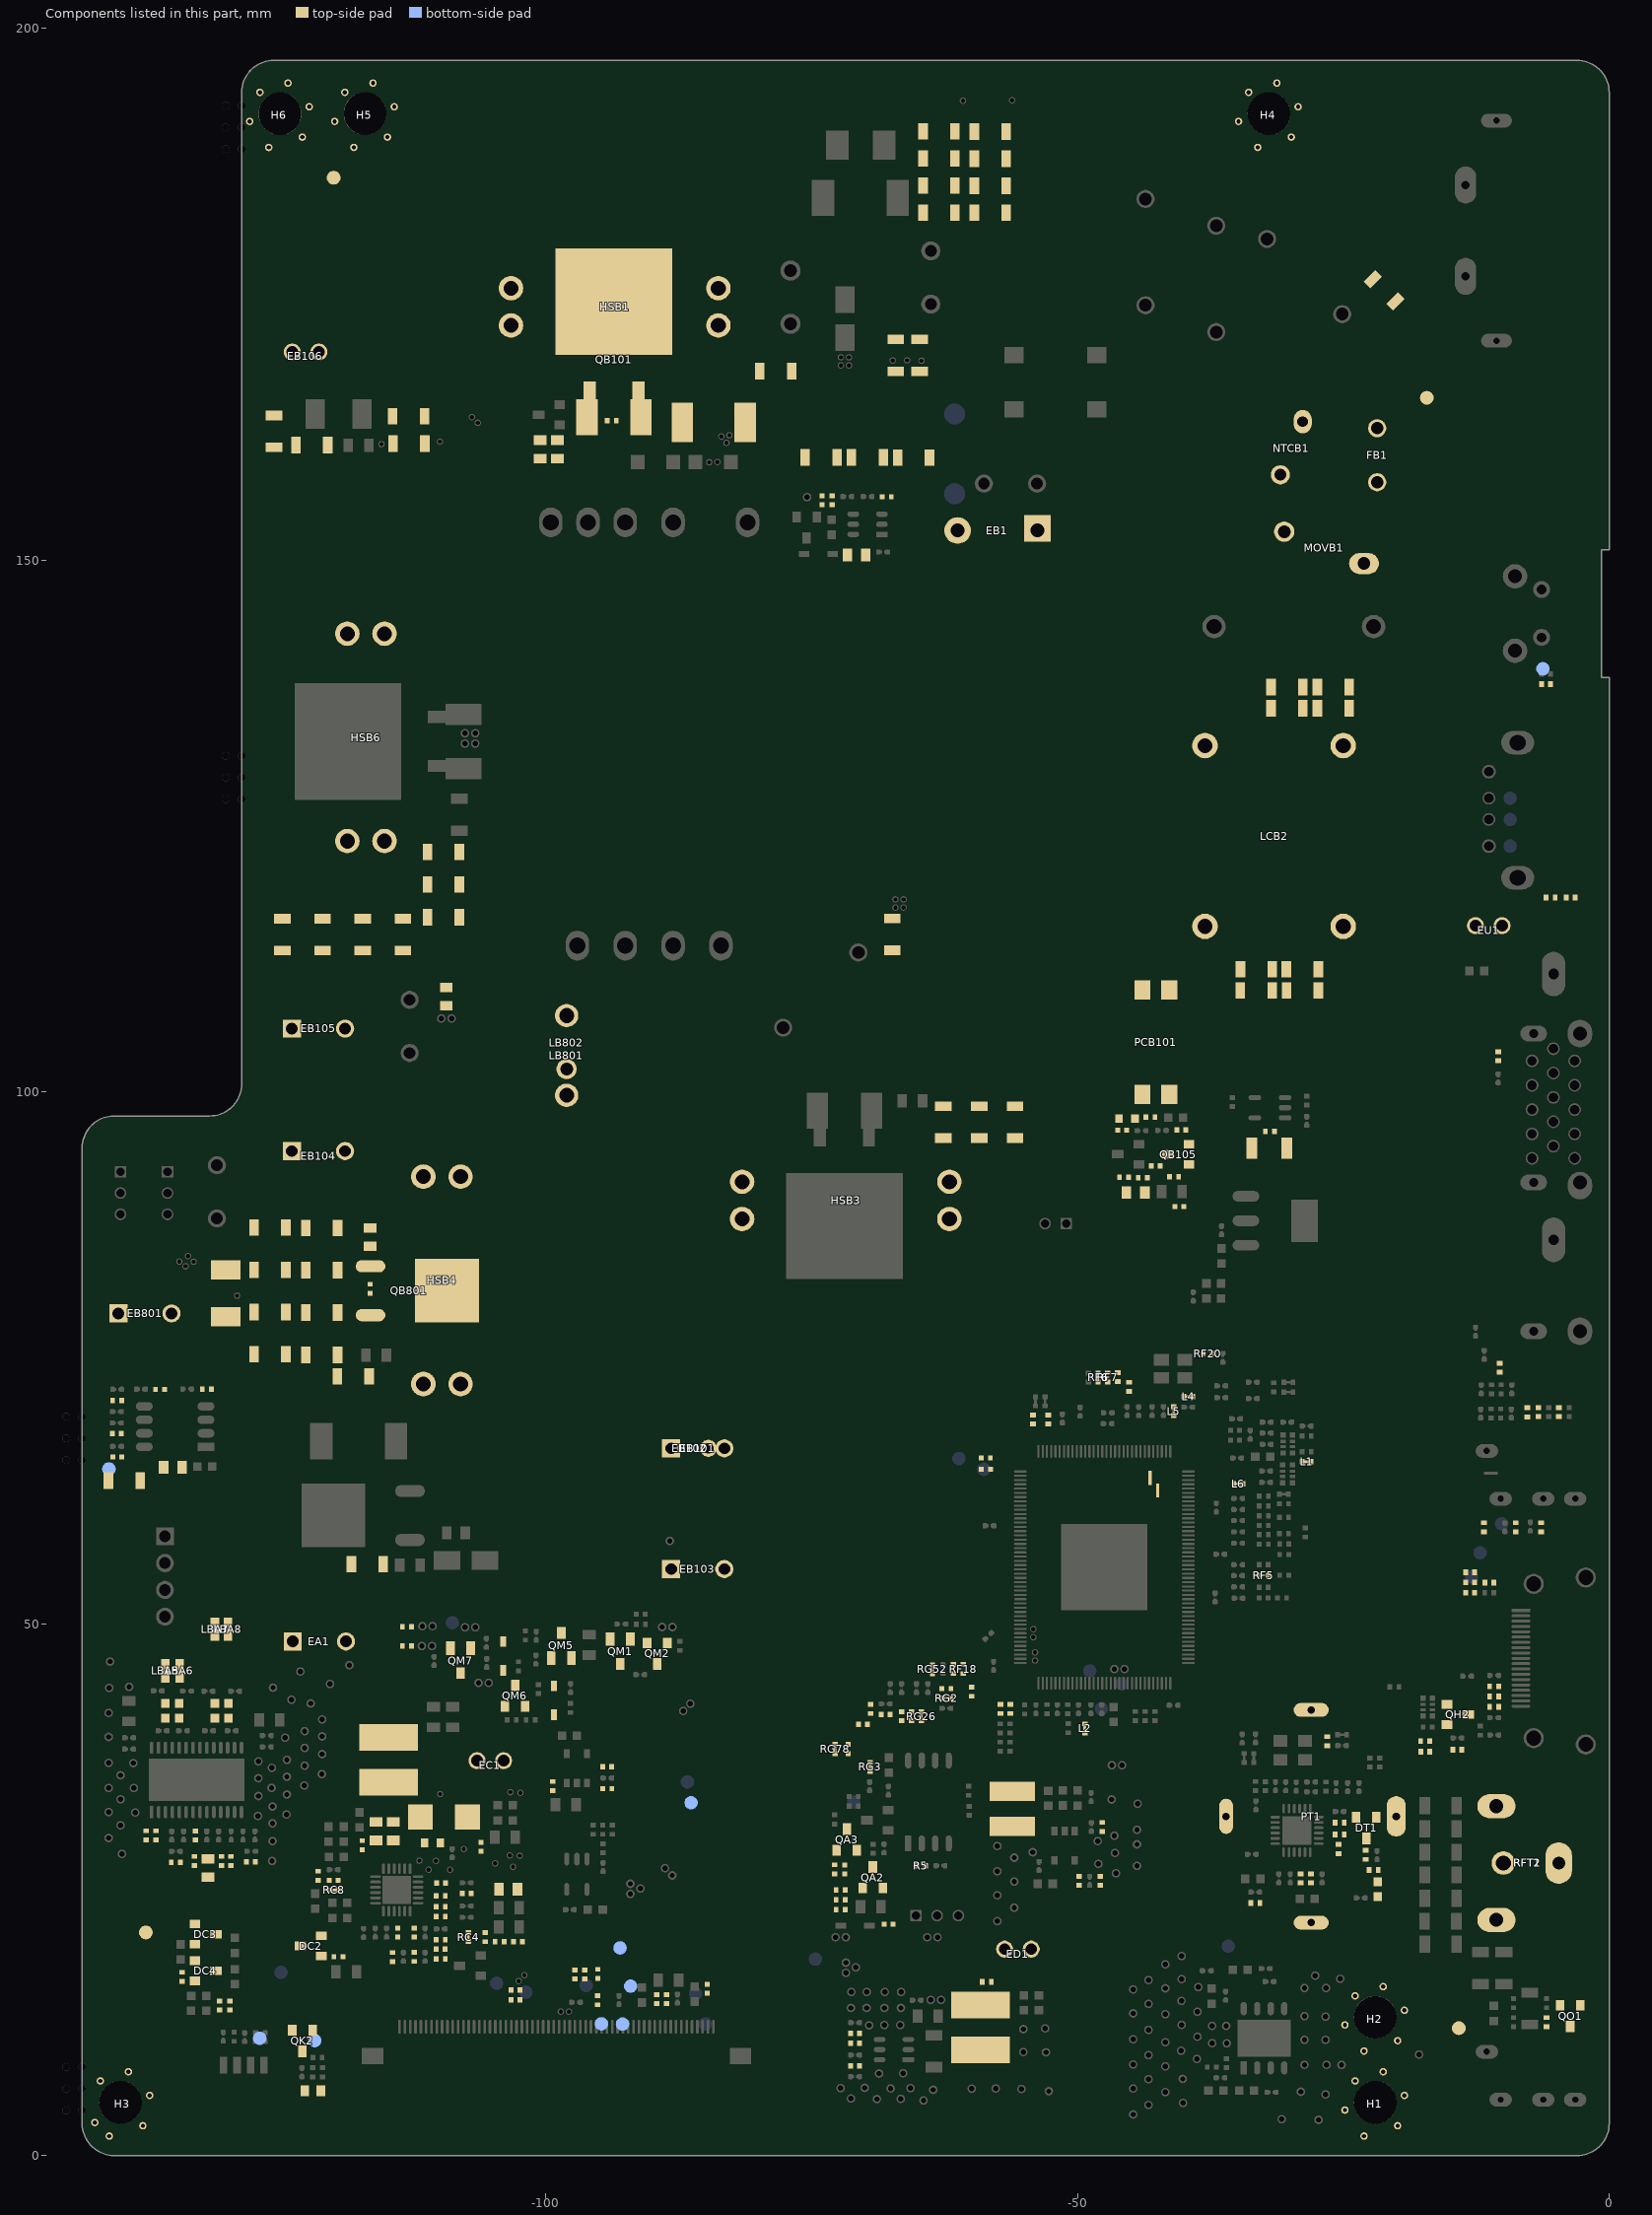
[diagram p0: the components of this part, seen from the top]
# Altium PCB MISC86383-9.PcbDoc (part 3 of 18)
Units mm, origin at the board's own origin, x right, y up, seen from the top; angles counter-clockwise.
Board outline 143.6 x 197 mm, 2 copper layers (TopLayer, BottomLayer), stack 1.571 mm thick; 743 components, 401 nets, 2996 pads, 1077 vias.
Unrouted connection lines stored in the file: 4.

## Components (designator, comment, footprint, x,y, rotation, side; value= is the part's Value field where it differs from the comment) (continued)
DB804 "Rectifier diode,DIO SI S,1A,1000V,SMAF,SMD,M7F,YJ" DIODE-S-2 -130.111,81.064 r270 top
DC1 "Schottky diode,DIO SBD S,1A,40V,DO-214AC,SMD,SS14W,WILLAS" DIODE-S-1 -109.576,31.826 r0 top
DC2 "Switching diode,DIO SW D2,200mA,100V,SOT-23,SMD,BAV99,YJ" SO-23 -122.117,19.704 r270 top
DC3 "Switching diode,DIO SW D2,200mA,100V,SOT-23,SMD,BAV99,YJ" SO-23 -131.977,20.816 r90 top
DC4 "Switching diode,DIO SW D2,200mA,100V,SOT-23,SMD,BAV99,YJ" SO-23 -131.989,17.368 r90 top
DH2 "NC/0ohm-0402-±5%-1/16W" DIODE-S0402 -13.074,52.916 r0 top
DH3 "NC/NC/AVLC18S02003" DIODE-S0402 -10.821,44.112 r0 top
DH6 "NC/NC/AVLC18S02003" DIODE-S0402 -10.821,43.147 r0 top
DH7 "NC/NC/AVLC18S02003" DIODE-S0402 -10.821,42.182 r0 top
DI1 "NC/AVLC18S02003" DIODE-S0402 -7.717,69.882 r90 top
DI2 "NC/AVLC18S02003" DIODE-S0402 -10.274,74.08 r90 top
DI3 "NC/AVLC18S02003" DIODE-S0402 -10.439,103.365 r270 top
DI5 "NC/NC/AVLC18S02003" DIODE-S0402 -5.893,12.543 r270 top
DK1 "TVS diode,DIO ESD,3pF,58V,0402,SMD,SDV1005H260C030YPTF,Sunlord" DIODE-S0402 -5.944,138.354 r0 top
DK2 "NC/TVS diode,DIO ESD,3pF,58V,0402,SMD,SDV1005H260C030YPTF,Sunlord" DIODE-S0402 -14.275,38.151 r180 top
DK6 "NC/TVS diode,DIO ESD,0.5pF,25V,0402 DFN,SMD,AZ5325-01F.R7G,Amazing" DIODE-S0402 -58.522,16.332 r0 top
DK20 "WEJT61RC-871-red" DIODE-S0603 -121.906,6.094 r0 top locked
DM1 "NC/Switching diode,DIO SW S,150mA,75V,SOD-323,SMD,1N4148WS,BLUE ROCKET" DIODE-S-12 -99.225,42.799 r270 top
DM3 "NC/Switching diode,DIO SW S,150mA,75V,SOD-323,SMD,1N4148WS,YJ" DIODE-S-12 -103.988,46.977 r270 top
DO1 "NC/AVLC18S02003" DIODE-S0402 -8.788,59.08 r90 top
DO2 "NC/AVLC18S02003" DIODE-S0402 -11.786,59.08 r90 top
DO3 "NC/AVLC18S02003" DIODE-S0402 -6.401,59.08 r90 top
DR1 "NC/AVLC18S02003" DIODE-S0402 -59.957,43.612 r90 top
DT1 "Switching diode,DIO SW D2,200mA,100V,SOT-23,SMD,BAV99,YJ" SO-23 -22.839,30.788 r0 top
DT2 "NC/AVLC18S02003" DIODE-S0402 -45.148,72.288 r90 top
DT3 "NC/AVLC18S02003" DIODE-S0402 -46.215,73.19 r90 top
DU1 "NC/" DIODE-S0402 -54.204,69.208 r270 top
DU2 "NC/" DIODE-S0402 -52.73,69.208 r270 top
DU3 "NC/" DIODE-S0402 -5.504,118.305 r0 top
DU4 "NC/" DIODE-S0402 -3.624,118.307 r180 top
DV1 "NC/SFI0402-240E-2R5PP-LF" DIODE-S0402 -56.297,41.99 r270 top
DV2 "NC/SFI0402-240E-2R5PP-LF" DIODE-S0402 -57.262,41.99 r270 top
DV3 "NC/NC/AVLC18S02003" DIODE-S0402 -11.26,53.861 r180 top
DV4 "NC/NC/AVLC18S02003" DIODE-S0402 -13.074,54.847 r0 top
DV5 "NC/SFI0402-240E-2R5PP-LF" DIODE-S0402 -4.724,69.901 r270 top
DV6 "NC/SFI0402-240E-2R5PP-LF" DIODE-S0402 -6.655,69.901 r270 top
DV7 "NC/SFI0402-240E-2R5PP-LF" DIODE-S0402 -17.306,38.969 r0 top
DV8 "NC/SFI0402-240E-2R5PP-LF" DIODE-S0402 -17.29,37.952 r0 top
DVDD "TEST" TP -93.015,19.52 r180 bottom
EA1 "Aluminium electrolytic capacitor,CAP AL,16V,470uF,±20%,PKRM,P,5.0mm,10×12.5,DIP,TP,Koshin" EC(10*12.5)-V-5#1 -121.298,48.336 r0 top locked
EB1 "Aluminium electrolytic capacitor,CAP AL,450V,82uF,±20%,SL,KL,BK,7.5mm,18×35.5,DIP,CapXon" EC(18*36)-H7.5-1 -57.525,152.801 r0 top locked
EB101 "Aluminium electrolytic capacitor,CAP AL,25V,470uF,±20%,LD,GK,P,5.0mm,10×12.5,DIP,TP,Samxon" EC(10*12.5)-V-5#2 -85.712,66.497 r0 top
EB102 "NC/270uF-16V-±20%-8×11-105℃-RP-short lead-F=3.5(Elite)" EC(8*11)-V-3.5 -86.462,66.497 r0 top
EB103 "NC/Aluminium electrolytic capacitor,CAP AL,25V,470uF,±20%,LD,GK,P,5.0mm,10×12.5,DIP,TP,Samxon" EC(10*12.5)-V-5#3 -85.712,55.143 r0 top
EB104 "Aluminium electrolytic capacitor,CAP AL,35V,330uF,±20%,LD,PKZF,P,5.0mm,10×12.5,DIP,TP,Koshin" EC(10*12.5)-V-5#4 -121.374,94.45 r0 top
EB105 "Aluminium electrolytic capacitor,CAP AL,35V,330uF,±20%,LD,PKZF,P,5.0mm,10×12.5,DIP,TP,Koshin" EC(10*12.5)-V-5#5 -121.374,105.969 r0 top
EB106 "Aluminium electrolytic capacitor,CAP AL,50V,10uF,±20%,LF,GH,P,2.5mm,5×11,DIP,TP,CapXon" EC(5*11)-V-2.5 -122.593,169.583 r0 top
EB801 "Aluminium electrolytic capacitor,CAP AL,63V,100uF,±20%,LD,GF,P,5.0mm,10×12.5,DIP,TP,CapXon" EC(10*12.5)-V-5#6 -137.693,79.184 r0 top locked
EC1 "Aluminium electrolytic capacitor,CAP AL,35V,100uF,±20%,LD,KF,P,2.5mm,6.3×11,DIP,TP,CapXon" EC(6.3*11)-V-2.5#1 -105.219,37.122 r0 top locked
ED1 "Aluminium electrolytic capacitor,CAP AL,10V,470uF,±20%,PKZH,P,2.5mm,6.3×11,DIP,TP,Koshin" EC(6.3*11)-V-2.5#2 -55.601,19.406 r0 top
EU1 "NC/Aluminium electrolytic capacitor,CAP AL,10V,470uF,±20%,PKZH,P,2.5mm,6.3×11,DIP,TP,Koshin" EC(6.3*11)-V-2.5#3 -11.328,115.646 r0 top
EVA1 "NC/7×7×3mm-C-4305 fire-retardant foam-black" EVA(7*7*3) 16.883,173.525 r0 top
EVA2 "NC/7×7×3mm-C-4305 fire-retardant foam-black" EVA(7*7*3) 26.01,173.525 r0 top
EVA3 "NC/7×7×3mm-C-4305 fire-retardant foam-black" EVA(7*7*3) 16.883,182.652 r0 top
EVA4 "NC/7×7×3mm-C-4305 fire-retardant foam-black" EVA(7*7*3) -48.133,5.842 r180 bottom
EVA5 "NC/7×7×3mm-C-4305 fire-retardant foam-black" EVA(7*7*3) -18.288,95.758 r180 bottom
EVA6 "NC/7×7×3mm-C-4305 fire-retardant foam-black" EVA(7*7*3) -136.779,33.655 r180 bottom
F2 "Thick film resistor,RES,1/16W,0ohm,±1%,0402,SMD" R0402#1 -31.902,96.291 r0 top
FB1 "Slow-blow fuse,FUSE T,P,3.15A,250VAC,8.5×4.0×8mm,DIP,TP,Walter" "FUSE8.5*4-V-5(T3.15AL 250V~)" -21.819,159.88 r90 top
FU1 "NC/NSMD110(1206-1.1A)" FUSE1.1A-S -31.953,94.717 r180 top
GD1 "NC/Mylar sheet spacer post,nylon,7.00×8.35mm,white,WQM" Fixed -123,178 r0 top locked
GD2 "NC/Mylar sheet spacer post,nylon,7.00×8.35mm,white,WQM" Fixed -4.813,155.207 r0 top
GD3 "NC/Mylar sheet spacer post,nylon,7.00×8.35mm,white,WQM" Fixed -86,104 r0 top locked
GL1 "Silicone,0.5g,general,60,white,SLD-8854W,XY" "Silica gel-20" -97.993,225.222 r180 top
GL2 "NC/Silicone,0.5g,general,60,white,SLD-8854W,XY" "Silica gel-10" 27.636,212.133 r0 top
GL3 "NC/Silicone,0.5g,general,60,white,SLD-8854W,XY" "Silica gel-10" 15.382,202.006 r0 top
GL4 "NC/Silicone,0.5g,general,60,white,SLD-8854W,XY" "Silica gel-10" 21.509,212.133 r0 top
GL5 "NC/Silicone,0.5g,general,60,white,SLD-8854W,XY" "Silica gel-10" 15.382,212.133 r0 top
GREF "TEST" TP -92.024,15.926 r180 bottom
H1 "Location hole" ASSE4.0C-3#1 -22,5 r0 top locked
H2 "Location hole" ASSE4.0C-3#1 -22,13 r0 top locked
H3 "Location hole" ASSE4.0C-3#2 -140,5 r0 top locked
H4 "Location hole" ASSE4.0C-3#1 -32,192 r0 top locked
H5 "Location hole" ASSE4.0C-3#1 -117,192 r0 top locked
H6 "Location hole" ASSE4.0C-3#1 -125,192 r0 top locked
"High Voltage" "High Voltage" "High Voltage" -175.59,208.28 r0 top
HS1 "Heat sink,aluminium alloy,18.8×13.8×5.0mm,natural,LHD" HS(18.8*13.8*5) -47.471,55.313 r0 top locked
HS2 "NC/Heat sink,15.0×15.0×5.0mm,AL1060H-24,black,high-emissivity paint,stamped with bend,no press-fit legs,YT" HS(15X15X5)-S -47.471,55.313 r0 top locked
HSB1 "NC/Heat sink,cold-rolled plate,natural,20×12×8.5mm,0.1k/W,bright tin plated,200mm2,1W,DIP PIN,TO-263,MRD" HS151 -93.523,173.838 r180 top
HSB3 "NC/Heat sink,cold-rolled plate,natural,20×12×8.5mm,0.1k/W,bright tin plated,200mm2,1W,DIP PIN,TO-263,MRD" HS151 -71.793,89.814 r0 top
HSB4 "NC/Heat sink,cold-rolled plate,natural,20×12×8.5mm,0.1k/W,bright tin plated,200mm2,1W,DIP PIN,TO-263,MRD" HS151 -109.766,82.296 r270 top
HSB6 "NC/Heat sink,cold-rolled plate,natural,20×12×8.5mm,0.1k/W,bright tin plated,200mm2,1W,DIP PIN,TO-263,MRD" HS151 -116.916,133.35 r90 top
IR "TEST" TP -126.905,11.025 r270 bottom
KEY "TEST" TP -6.236,139.802 r270 bottom
L1 "NC/0ohm-0402-PCB" R0402SC -28.443,65.23 r180 top
L2 "NC/0ohm-0402-PCB" R0402SC -49.312,40.162 r90 top
L4 "NC/0ohm-0402-PCB" R0402SC -39.573,71.374 r0 top
L5 "NC/0ohm-0402-PCB" R0402SC -40.959,69.989 r270 top
L6 "NC/0ohm-0402-PCB" R0402SC -34.874,63.17 r180 top
LB801 "Differential-mode inductor,Inductor,DR12×12,70uH,0.15×12P,38.5Ts,H13.5MAX,SYDR1212-L070uA,DIP,DL" L/LC2/15*14.5-V7.5 -98.044,103.441 r270 top
LB802 "NC/Differential-mode inductor,Inductor,DR12×14,68uH,0.45,20Ts,H13.5MAX,SYDR1214-L068uA,DIP,Soldier" L(13.5*15.5)-V-5 -98.044,104.661 r270 top
LBA1 "Ferrite bead,BEAD,600ohm,0603,2A,SMD,TP,EPZ1608E601-2R0TF,Sunlord" L0603 -135.791,41.818 r90 top
LBA2 "Ferrite bead,BEAD,600ohm,0603,2A,SMD,TP,EPZ1608E601-2R0TF,Sunlord" L0603 -134.471,41.818 r90 top
LBA3 "Ferrite bead,BEAD,600ohm,0603,2A,SMD,TP,EPZ1608E601-2R0TF,Sunlord" L0603 -131.123,41.818 r90 top
LBA4 "Ferrite bead,BEAD,600ohm,0603,2A,SMD,TP,EPZ1608E601-2R0TF,Sunlord" L0603 -129.848,41.818 r90 top
LBA5 "NC/0ohm-0603-PCB" R0603SC -135.791,45.578 r90 top
LBA6 "NC/0ohm-0603-PCB" R0603SC -134.42,45.578 r90 top
LBA7 "NC/0ohm-0603-PCB" R0603SC -131.118,49.489 r90 top
LBA8 "NC/0ohm-0603-PCB" R0603SC -129.899,49.489 r90 top
LC1 "Power inductor,Power Inductor,10uH,±10%,2A,0.3×1P,DR5.8×4.5,SMD,CKO54-10uH/K,CK" L(5.8*4.5)-S -114.795,37.224 r90 top
LCB2 "Common-mode choke,Common Choke,UC1614,10.5mH±10%,0.15×1.0mm,48Ts,H14.0MAX,SYUC16-L10.5mA,DIP,CH" L/LC4/21*17-H-17*13 -31.509,124.079 r90 top
LD1 "Power inductor,Power Inductor,4.7uH,±20%,2.8A,0.32×1P,DR5.8×4.5,SMD,PIO54-4R7MTP02,FH" L(5.8*4.5)-S -59.106,12.04 r270 top
LD2 "Power inductor,Power Inductor,2.2uH,±20%,2A,0.28×1P,DR4.5×3.2,SMD,PIO43-2R2MTP02,FH" L(4.5*3.5)-S -56.134,32.587 r270 top
LED "TEST" TP -121.729,10.808 r270 bottom
LF1 "1000pF-0402-X7R-±10%-50V" L0402 -26.519,38.966 r90 top
LT1 "Multilayer inductor,HF Inductor,68nH,±5%,0402,SMD,SDCL1005C68NJTDF,Sunlord" L0402 -28.064,26.062 r90 top
LT2 "GZ1005U102CTF(1000ohm-300mA)" L0402 -29.029,26.063 r270 top
LT3 "Thick film resistor,RES,1/16W,0ohm,±1%,0402,SMD" L0402 -22.906,28.272 r90 top
LT6 "GZ1005U102CTF(1000ohm-300mA)" L0402 -25.435,28.818 r270 top
LT8 "GZ1005U102CTF(1000ohm-300mA)" L0402 -25.346,30.177 r0 top
LT9 "NC/SDCL1608CR22JT(F)" L0603 -21.75,25.04 r270 top
LT10 "SDCL1005CR18JTDF(180nH-0402±5%-C)" L0402 -25.346,31.282 r0 top
LT11 "NC/SDCL1005CR27JTDF(Sunlord)" L0402 -22.146,26.839 r180 top
LT12 "Ferrite bead,BEAD,120ohm,0402,800mA,SMD,TP,CBM100505U121T,FH" L0402 -33.263,23.726 r0 top
M1 "MARK" MARK -17.145,165.278 r0 top
M2 "MARK" MARK -119.951,185.979 r0 top
M3 "MARK" MARK -137.615,20.977 r0 top
M4 "MARK" MARK -14.142,11.976 r0 top
Manufacture_Info "Manufacture_Info" Manufacture_Info -21.537,56.697 r180 top
ML1 "NC/Mylar sheet,XXXXXXXXXXXXXXX,(85+6)×(123.5+6)×0.43mm,SE42B,black" Mylar 19.761,164.897 r90 top
MOVB1 "Varistor,VARISTOR,128J,680V,4000A,S,7.5mm,10mm,DIP,Thinking" VR(13*5)-V-7.5 -26.81,151.193 r0 top
"NO DOLBY" "NO DOLBY" "NO DOLBY-SILK" -43.815,53.213 r180 bottom
NTCB1 "SCK102R55AMBY502(short lead/Weiqin)" NTC(10*5)-V5 -29.87,160.541 r90 top
OE1 "TEST" TP -86.335,33.172 r180 bottom
PCB101 "LTV-817S-TA-B(Lite-On)" OC4-S-1 -42.634,104.686 r0 top
PCB101及周围贴片器件 "NC/Conformal coating,25kg/Can,Peters" PCB_TIME 34.45,168.811 r90 top
POL "TEST" TP -94.767,12.383 r180 bottom
PT1 "20.3×16.3×6-LHD (with seal)" SHIELD(16*20*6) -28.026,21.897 r0 top locked
PWM_REF "NC/TEST" TP_BL -141.084,64.554 r180 bottom
QA2 "NC/LMBT3906LT1G" SOT-23 -69.258,26.173 r180 top
QA3 "NC/LMBT3904LT1G" SOT-23 -71.696,29.729 r180 top
QB101 "MOSFET,NMOS,8A,650V,0.48ohm@ID=4A@VGS=10V,TO-252,OSG65R580DEF,ORIENTAL SEMICONDUCTOR" D2PAK3 -93.688,170.955 r270 top
QB105 "NC/General transistor,Dynatron,NPN,0.2A,40V,30-300,SOT-23,LMBT3904LT1G,LRC" SOT-23 -40.538,94.132 r270 top
QB801 "MOSFET,NMOS,15A,100V,0.105ohm@ID=6A@VGS=10V,TO-252,PA110BDA,UNIKC" TO-252-GDS -109.283,81.318 r270 top
QH2 "General transistor,Dynatron,NPN,0.2A,40V,30-300,SOT-23,LMBT3904LT1G,LRC" SOT-23 -14.225,41.471 r90 top
QK2 "NC/MMBT3904(f≥350MHz)" SOT-23 -122.885,10.77 r0 top
QM1 "MOSFET,PMOS,-4.4A,-30V,0.046ohm@ID=-4A@VGS=-4.5V,SOT-23,NCE3401AY,NCEPOWER" SOT-23-1 -93.003,47.371 r0 top
QM2 "General transistor,Dynatron,NPN,0.2A,40V,30-300,SOT-23,LMBT3904LT1G,LRC" SOT-23 -89.522,47.18 r0 top
QM5 "MOSFET,PMOS,-4.4A,-30V,0.046ohm@ID=-4A@VGS=-4.5V,SOT-23,NCE3401AY,NCEPOWER" SOT-23-1 -98.54,47.981 r180 top
QM6 "General transistor,Dynatron,NPN,0.2A,40V,30-300,SOT-23,LMBT3904LT1G,LRC" SOT-23 -102.895,43.243 r180 top
QM7 "MOSFET,PMOS,-4.3A,-30V,0.048ohm@ID=-3A@VGS=-4.5V,SOT-23-3L,NCE3407AY,NCEPOWER" SOT-23-1 -108.013,46.507 r0 top
QO1 "NC/General transistor,Dynatron,NPN,0.2A,40V,60-300,SOT-23,KMBT3904,KEXIN" SOT-23 -3.658,13.102 r0 top
R5 "Thick film resistor,RES,1/16W,10Kohm,±1%,0402,SMD" R0402#2 -64.712,27.254 r180 top
RA1 "Thick film resistor,RES,1/16W,4.7Kohm,±1%,0402,SMD" R0402#1 -137.578,30.109 r270 top
RA2 "NC/" GND -42.456,62.535 r90 top
RA3 "Thick film resistor,RES,1/8W,10ohm,±1%,0805,SMD" R0805 -131.783,27.036 r90 top
RA4 "NC/100Kohm-0402-±5%-1/16W" R0402#1 -133.048,27.696 r270 top
RA5 "Thick film resistor,RES,1/16W,1Kohm,±1%,0402,SMD" R0402#1 -127.728,27.602 r0 top
RA8 "Thick film resistor,RES,1/16W,4.7Kohm,±1%,0402,SMD" R0402#1 -136.657,30.103 r90 top
RA10 "NC/2K2ohm-0402-±5%-1/16W" R0402#1 -71.89,26.897 r90 top
RA11 "NC/10Kohm-0402-±1%-1/16W" R0402#1 -130.512,27.696 r90 top
RA12 "NC/15Kohm-0402-±1%-1/16W" R0402#1 -129.598,27.696 r90 top
RA14 "NC/0ohm-0402-±5%-1/16W" R0402#1 -132.947,30.084 r90 top
RA15 "NC/" GND -43.18,63.716 r90 top
RA16 "NC/2Kohm-0402-±1%-1/16W" R0402#1 -72.28,24.04 r0 top
RA18 "NC/33Kohm-0402-±5%-1/16W" R0402#1 -72.28,23.125 r180 top
RA19 "NC/33Kohm-0402-±5%-1/16W" R0402#1 -72.28,24.98 r180 top
RA21 "Thick film resistor,RES,1/16W,1Kohm,±1%,0402,SMD" R0402#1 -134.798,27.584 r0 top
RA31 "NC/NC/470Kohm-0402-±5%-1/16W" R0402#1 -67.759,21.754 r180 top
RA38 "NC/100Kohm-0402-±5%-1/16W" R0402#1 -72.83,26.909 r90 top
RB1 "1M2ohm-1206-±5%-1/4W" R1206 -25.946,136.08 r180 top
RB2 "1M2ohm-1206-±5%-1/4W" R1206 -25.946,138.087 r180 top
RB3 "1M2ohm-1206-±5%-1/4W" R1206 -30.302,136.08 r180 top
RB4 "1M2ohm-1206-±5%-1/4W" R1206 -30.302,138.087 r180 top
RB101 "Thick film resistor,RES,1/4W,510Kohm,±1%,1206,SMD" R1206 -28.842,109.563 r180 top
RB101,102,143,144电阻附近 "NC/Conformal coating,25kg/Can,Peters" PCB_TIME 34.75,168.811 r90 top
RB102 "Thick film resistor,RES,1/4W,510Kohm,±1%,1206,SMD" R1206 -33.185,109.563 r180 top
RB103 "Thick film resistor,RES,1/16W,3Kohm,±1%,0402,SMD" R0402#1 -73.076,155.651 r90 top
RB104 "NC/Thick film resistor,RES,1/16W,30Kohm,±1%,0402,SMD" R0402#1 -67.932,155.969 r180 top
RB105 "Thick film resistor,RES,1/16W,510ohm,±1%,0402,SMD" R0402#1 -74.016,155.638 r270 top
RB106 "Thick film resistor,RES,1/8W,68ohm,±5%,0805,SMD" R0805 -98.92,160.439 r90 top
RB107 "Thick film resistor,RES,1/8W,20ohm,±5%,0805,SMD" R0805 -100.546,160.426 r90 top
RB109 "Thick film resistor,RES,1/16W,10Kohm,±1%,0402,SMD" R0402#1 -93.789,163.144 r180 top
RB110 "0ohm-1206-±5%-1/4W" R1206 -125.565,162.115 r90 top
RB112 "Thick film resistor,RES,1/8W,24Kohm,±1%,0805,SMD" R0805 -70.777,150.482 r180 top
RB114 "Thick film resistor,RES,1/4W,4.7ohm,±1%,1206,SMD" R1206 -112.878,160.972 r0 top
RB115 "NC/4R7ohm-1206-±1%-1/4W" R1206 -112.903,163.538 r0 top
RB116 "NC/10ohm-1206-±5%-1/4W" R1206 -122.009,160.845 r180 top
RB117 "Thick film resistor,RES,1/4W,10ohm,±1%,1206,SMD" R1206 -64.833,169.278 r270 top
RB118 "Thick film resistor,RES,1/4W,10ohm,±1%,1206,SMD" R1206 -67.081,169.278 r270 top
RB119 "Thick film resistor,RES,1/4W,10ohm,±1%,1206,SMD" R1206 -78.372,167.78 r0 top
RB124 "68ohm-1206-±5%-1/4W" R1206 -120.997,114.795 r90 top
RB125 "68ohm-1206-±5%-1/4W" R1206 -109.626,122.58 r180 top
RB126 "68ohm-1206-±5%-1/4W" R1206 -109.626,116.446 r180 top
RB127 "68ohm-1206-±5%-1/4W" R1206 -117.217,114.795 r90 top
RB128 "Thick film resistor,RES,1/4W,47ohm,±5%,1206,SMD" R1206 -55.88,97.168 r270 top
RB129 "Thick film resistor,RES,1/4W,47ohm,±5%,1206,SMD" R1206 -62.611,97.168 r270 top
RB130 "Thick film resistor,RES,1/4W,20ohm,±1%,1206,SMD" R1206 -67.424,114.833 r270 top
RB131 "Thick film resistor,RES,1/10W,2Kohm,±1%,0603,SMD" R0603 -45.346,97.511 r180 top
RB132 "Thick film resistor,RES,1/16W,1.2Kohm,±1%,0402,SMD" R0402#1 -43.136,97.638 r180 top
RB133 "Thick film resistor,RES,1/16W,10Kohm,±1%,0402,SMD" R0402#1 -40.234,96.444 r0 top
RB134 "Thick film resistor,RES,1/16W,5.1Kohm,±1%,0402,SMD" R0402#1 -43.866,91.948 r180 top
RB135 "Thick film resistor,RES,1/16W,20Kohm,±1%,0402,SMD" R0402#1 -45.618,91.973 r0 top
RB140 "Thick film resistor,RES,1/8W,51Kohm,±1%,0805,SMD" R0805 -109.36,108.979 r90 top
RB141 "NC/Thick film resistor,RES,1/4W,2Mohm,±5%,1206,SMD" R1206 -28.854,111.557 r0 top
RB142 "NC/Thick film resistor,RES,1/4W,2Mohm,±5%,1206,SMD" R1206 -33.172,111.544 r0 top
RB143 "NC/Thick film resistor,RES,1/4W,2Mohm,±5%,1206,SMD" R1206 -65.418,159.664 r0 top
RB144 "NC/Thick film resistor,RES,1/4W,2Mohm,±5%,1206,SMD" R1206 -69.761,159.677 r0 top
RB145 "NC/Thick film resistor,RES,1/4W,2Mohm,±5%,1206,SMD" R1206 -74.117,159.677 r0 top
RB148 "Thick film resistor,RES,2W,0.27ohm,±5%,2512,SMD" R2512-1 -84.201,162.979 r180 top
RB150 "150Kohm-1206-±5%-1/4W" R1206 -58.204,187.765 r0 top
RB151 "150Kohm-1206-±5%-1/4W" R1206 -58.204,190.309 r0 top
RB152 "150Kohm-1206-±5%-1/4W" R1206 -58.204,182.677 r0 top
RB153 "150Kohm-1206-±5%-1/4W" R1206 -63.017,182.677 r0 top
RB154 "150Kohm-1206-±5%-1/4W" R1206 -63.017,185.229 r0 top
RB155 "150Kohm-1206-±5%-1/4W" R1206 -63.017,190.335 r0 top
RB156 "NC/150Kohm-1206-±5%-1/4W" R1206 -58.204,185.221 r0 top
RB157 "NC/150Kohm-1206-±5%-1/4W" R1206 -63.017,187.782 r0 top
RB158 "NC/Thick film resistor,RES,1/16W,51ohm,±1%,0402,SMD" R0402#1 -45.796,96.418 r180 top
RB160 "Thick film resistor,RES,1/4W,20ohm,±1%,1206,SMD" R1206 -21.158,175.387 r135 top
RB162 "NC/68ohm-1206-±5%-1/4W" R1206 -109.626,119.513 r180 top
RB163 "NC/68ohm-1206-±5%-1/4W" R1206 -124.777,114.795 r90 top
RB164 "NC/68ohm-1206-±5%-1/4W" R1206 -113.436,114.795 r90 top
RB165 "NC/68ohm-1206-±5%-1/4W" R1206 -59.245,97.168 r270 top
RB180 "NC/Thick film resistor,RES,1/16W,18Kohm,±1%,0402,SMD" R0402#1 -42.647,93.066 r180 top
RB181 "NC/1Kohm-0805-±1%-1/8W" R0805 -44.526,90.551 r0 top
RB182 "NC/Thick film resistor,RES,1/16W,4.7Kohm,±1%,0402,SMD" R0402#1 -40.411,89.23 r180 top
RB183 "NC/Thick film resistor,RES,1/16W,10Kohm,±1%,0402,SMD" R0402#1 -40.919,92.024 r180 top
RB803 "Thick film resistor,RES,1/16W,10Kohm,±1%,0402,SMD" R0402#1 -140.345,67.894 r0 top
RB804 "NC/10Kohm-0402-±5%-1/16W" R0402#1 -140.316,70.98 r0 top
RB805 "Thick film resistor,RES,1/16W,100ohm,±1%,0402,SMD" R0402#1 -136.278,72.038 r0 top
RB806 "Thick film resistor,RES,1/16W,1Kohm,±1%,0402,SMD" R0402#1 -131.883,72.074 r0 top
RB807 "20ohm-0805-±5%-1/8W" R0805 -116.522,86.36 r270 top
RB808 "10Kohm-0402-±1%-1/16W" R0402#1 -116.522,81.509 r90 top
RB810 "Thick film resistor,RES,1/4W,10ohm,±1%,1206,SMD" R1206 -118.11,73.266 r180 top
RB812 "Thick film resistor,RES,1/4W,10ohm,±1%,1206,SMD" R1206 -116.789,55.613 r180 top
RB813 "Thick film resistor,RES,1/16W,100ohm,±1%,0402,SMD" R0402#1 -140.294,65.684 r180 top
RB814 "Thick film resistor,RES,1/4W,270Kohm,±1%,1206-Auto,SMD" R1206 -139.636,63.462 r0 top
RB816 "Thick film resistor,RES,1/8W,10ohm,±1%,0805,SMD" R0805 -135.064,64.706 r0 top
RB818 "Thick film resistor,RES,1/4W,0.2ohm,±1%,1206,SMD" R1206 -121.082,79.265 r180 top
RB819 "Thick film resistor,RES,1/4W,0.2ohm,±1%,1206,SMD" R1206 -121.082,75.286 r180 top
RB820 "Thick film resistor,RES,1/4W,0.2ohm,±1%,1206,SMD" R1206 -121.082,87.224 r180 top
RB821 "Thick film resistor,RES,1/4W,0.2ohm,±1%,1206,SMD" R1206 -121.082,83.244 r180 top
RB837 "Thick film resistor,RES,1/4W,2ohm,±1%,1206,SMD" R1206 -125.946,83.282 r180 top
RB838 "Thick film resistor,RES,1/4W,2ohm,±1%,1206,SMD" R1206 -125.946,79.316 r180 top
RB839 "Thick film resistor,RES,1/4W,2ohm,±1%,1206,SMD" R1206 -125.946,75.349 r0 top
RB840 "NC/1R5ohm-1206-±1%-1/4W" R1206 -125.946,87.249 r180 top
RC1 "33ohm-0805-±5%-1/8W" R0805 -103.53,25.044 r180 top
RC2 "12Kohm-0402-±1%-1/16W" R0402#1 -104.343,20.117 r0 top
RC3 "Thick film resistor,RES,1/16W,1.8Kohm,±1%,0402,SMD" R0402#1 -105.715,20.523 r270 top
RC4 "NC/0ohm-0402-PCB" R0402SC -107.29,20.523 r90 top
RC8 "NC/0ohm-0402-PCB" R0402SC -119.945,24.948 r0 top
RC10 "Thick film resistor,RES,1/16W,100Kohm,±1%,0402,SMD" R0402#1 -109.893,19.393 r0 top
RC12 "Thick film resistor,RES,1/16W,33Kohm,±1%,0402,SMD" R0402#1 -109.884,22.471 r180 top
RC13 "Thick film resistor,RES,1/16W,51Kohm,±1%,0402,SMD" R0402#1 -109.884,24.401 r0 top
RC14 "Thick film resistor,RES,1/16W,4.7ohm,±1%,0402,SMD" R0402#1 -109.88,20.304 r0 top
RC15 "Thick film resistor,RES,1/16W,47Kohm,±1%,0402,SMD" R0402#1 -109.884,23.385 r0 top
RC18 "Thick film resistor,RES,1/16W,47Kohm,±1%,0402,SMD" R0402#1 -106.096,29.02 r90 top
RC19 "NC/0ohm-0402-±5%-1/16W" R0402#1 -113.055,47.904 r0 top
RC20 "Thick film resistor,RES,1/16W,0ohm,±1%,0402,SMD" R0402#1 -113.055,49.733 r180 top
RC23 "NC/0ohm-0402-±5%-1/16W" R0402#1 -134.212,16.803 r270 top
RC24 "Thick film resistor,RES,1/16W,10Kohm,±1%,0402,SMD" R0402#1 -119.507,18.694 r180 top
RC27 "Thick film resistor,RES,1/16W,47Kohm,±1%,0402,SMD" R0402#1 -130.683,14.097 r270 top
RC31 "10Kohm-0402-±1%-1/16W" R0402#1 -94.221,36.551 r180 top
RC32 "Thick film resistor,RES,1/16W,0ohm,±1%,0402,SMD" R0402#1 -102.845,15.545 r180 top
RC33 "NC/0ohm-0402-±5%-1/16W" R0402#1 -102.845,14.631 r0 top
RC35 "10Kohm-0402-±1%-1/16W" R0402#1 -94.208,34.493 r0 top
RC36 "Thick film resistor,RES,1/16W,10ohm,±1%,0402,SMD" R0402#1 -99.365,34.747 r270 top
RD1 "Thick film resistor,RES,1/16W,100Kohm,±1%,0402,SMD" R0402#1 -70.92,8.435 r0 top
RD3 "Thick film resistor,RES,1/16W,60.4Kohm,±1%,0402,SMD" R0402#1 -70.918,11.474 r180 top
RD5 "Thick film resistor,RES,1/16W,10.5Kohm,±1%,0402,SMD" R0402#1 -70.918,10.56 r0 top
RD7 "Thick film resistor,RES,1/16W,100Kohm,±1%,0402,SMD" R0402#1 -47.689,30.897 r90 top
RD8 "Thick film resistor,RES,1/16W,13Kohm,±1%,0402,SMD" R0402#1 -49.851,25.82 r270 top
RD9 "Thick film resistor,RES,1/16W,12Kohm,±1%,0402,SMD" R0402#1 -47.865,25.82 r90 top
RF5 "NC/68ohm-0402-±5%-1/16W" R0402#2 -32.494,54.562 r0 top
RF6 "Thick film resistor,RES,1/16W,4.7Kohm,±1%,0402,SMD" R0402#2 -48.062,73.168 r90 top
RF7 "Thick film resistor,RES,1/16W,4.7Kohm,±1%,0402,SMD" R0402#2 -47.147,73.168 r90 top
RF13 "Thick film resistor,RES,1/16W,4.7Kohm,±1%,0402,SMD" R0402#1 -61.665,45.735 r270 top
RF14 "NC/4K7ohm-0402-±5%-1/16W" R0402#1 -62.332,43.901 r180 top
RF18 "Thick film resistor,RES,1/16W,4.7Kohm,±1%,0402,SMD" R0402#2 -60.754,45.743 r270 top
RF20 "Thick film resistor,RES,1/16W,1Kohm,±1%,0402,SMD" R0402#2 -37.755,75.417 r0 top
RFT1 "NC/RF connector,RF JACK,H,F,T14.5,CH6.3,without pipe,12.4×13.2×7.7mm,DIP,LHD" T-13.2×12.4×7.7-F14.5 -4.5,27.5 r90 top locked
RFT2 "RF connector,RF JACK,H,IEC,T14.5,CH6.3,12.4×13.2×7.7mm,DIP,LHD-020 assembly,LHD" ANT-IEC14.5-H-4 -4.5,27.5 r90 top locked
RG2 "NC/0ohm-0402-PCB" R0402SC -62.332,43.015 r0 top
RG3 "NC/0ohm-0402-PCB" R0402SC -69.52,36.551 r270 top
RG5 "Thick film resistor,RES,1/16W,0ohm,±1%,0402,SMD" R0402#1 -129.692,14.097 r270 top
RG6 "NC/0ohm-0402-±5%-1/16W" R0402#1 -117.259,29.185 r90 top
RG7 "Thick film resistor,RES,1/16W,10Kohm,±1%,0402,SMD" R0402#1 -95.11,17.081 r90 top
RG8 "Thick film resistor,RES,1/16W,470Kohm,±1%,0402,SMD" R0402#1 -107.444,24.632 r0 top
RG9 "Thick film resistor,RES,1/16W,75Kohm,±1%,0402,SMD" R0402#1 -114.399,18.664 r270 top
RG12 "NC/Thick film resistor,RES,1/16W,10Kohm,±1%,0402,SMD" R0402#1 -95.123,14.599 r270 top
RG13 "Thick film resistor,RES,1/16W,39Kohm,±1%,0402,SMD" R0402#1 -109.839,25.618 r180 top
RG14 "Thick film resistor,RES,1/16W,3Kohm,±1%,0402,SMD" R0402#1 -113.925,20.955 r90 top
RG15 "12Kohm-0402-±1%-1/16W" R0402#1 -121.405,26.307 r270 top
RG16 "10K5ohm-0402-±1%-1/16W" R0402#1 -119.953,25.875 r180 top
RG21 "49K9ohm-0402-±1%-1/16W" R0402#1 -112.376,18.669 r270 top
RG22 "6K2ohm-0402-±1%-1/16W" R0402#1 -112.376,20.955 r270 top
RG25 "NC/0ohm-0402-±5%-1/16W" R0402#1 -68.047,41.478 r180 top
RG26 "NC/0ohm-0402-PCB" R0402SC -64.694,41.3 r270 top
RG39 "Thick film resistor,RES,1/16W,0ohm,±1%,0402,SMD" R0402#1 -89.56,14.707 r90 top
RG40 "Thick film resistor,RES,1/16W,0ohm,±1%,0402,SMD" R0402#1 -65.608,41.3 r270 top
RG41 "NC/0ohm-0402-±5%-1/16W" R0402#1 -84.823,15.672 r270 top
RG42 "Thick film resistor,RES,1/16W,0ohm,±1%,0402,SMD" R0402#1 -96.342,17.031 r270 top
RG43 "Thick film resistor,RES,1/16W,0ohm,±1%,0402,SMD" R0402#1 -97.257,17.031 r270 top
RG44 "NC/0ohm-0402-±5%-1/16W" R0402#1 -88.633,14.707 r270 top
RG46 "NC/0ohm-0402-±5%-1/16W" R0402#1 -66.523,41.3 r270 top
RG48 "Thick film resistor,RES,1/16W,0ohm,±1%,0402,SMD" R0402#1 -102.616,20.117 r0 top
RG49 "10Kohm-0402-±1%-1/16W" R0402#1 -109.88,18.466 r0 top
RG52 "NC/0ohm-0402-PCB" R0402SC -63.64,45.72 r270 top
RG58 "NC/Thick film resistor,RES,1/8W,1Kohm,±1%,0805,SMD" R0805 -115.976,30.493 r90 top
RG59 "Thick film resistor,RES,1/16W,0ohm,±1%,0402,SMD" R0402#1 -70.18,40.538 r180 top
RG60 "NC/33ohm-0402-±5%-1/16W" R0402#1 -58.61,64.529 r180 top
RG61 "NC/33ohm-0402-±5%-1/16W" R0402#1 -58.623,65.596 r180 top
RG62 "Thick film resistor,RES,1/16W,0ohm,±1%,0402,SMD" R0402#1 -69.469,41.986 r270 top
RG63 "NC/Thick film resistor,RES,1/8W,1Kohm,±1%,0805,SMD" R0805 -114.351,30.493 r90 top
RG78 "NC/0ohm-0402-PCB" R0402SC -72.784,38.227 r270 top
RG82 "Thick film resistor,RES,1/10W,22ohm,±1%,0603,SMD" R0603 -110.655,29.4 r180 top
RGV1 "NC/0ohm-0402-±5%-1/16W" R0402#1 -71.564,38.227 r270 top
RH1 "Thick film resistor,RES,1/16W,0ohm,±1%,0402,SMD" R0402#1 -13.074,53.882 r0 top